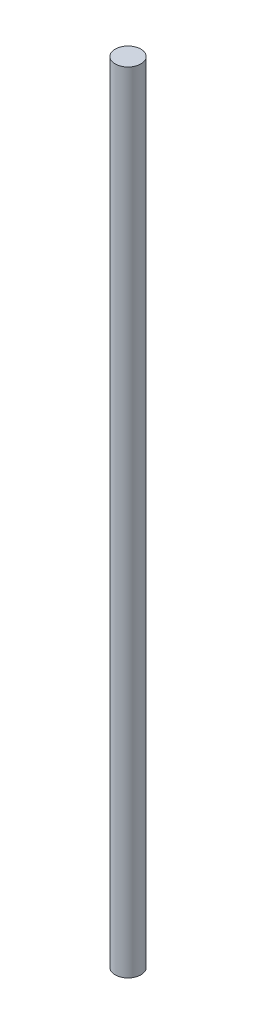
from build123d import *

# Parameters (mm, degrees)
SKETCH1_W = 1.5
SKETCH1_H = 92


with BuildPart() as part:
    # Sketch1 → Revolve1 (revolve)
    with BuildSketch(Plane.XY, mode=Mode.PRIVATE) as revolve1_sk:
        with Locations((0.75, 46)):
            Rectangle(SKETCH1_W, SKETCH1_H)
    revolve(revolve1_sk.sketch.rotate(Axis((0, 0, 0), (0, 1, 0)), 90), axis=Axis((0, 0, 0), (0, 1, 0)))


solid = part.part
